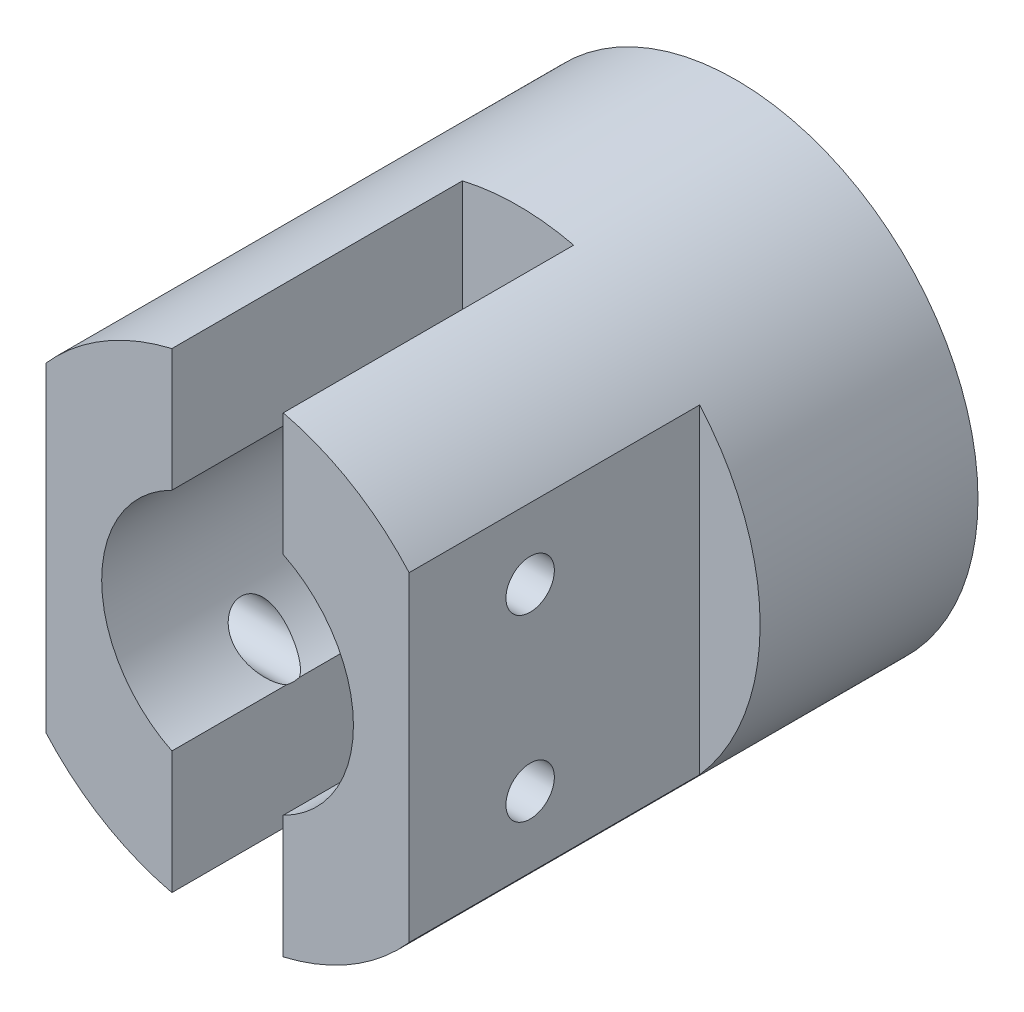
from build123d import *

# Parameters (mm, degrees)
SKETCH2_R           = 5
BOSS_EXTRUDE1_DEPTH = 10.5
SKETCH3_R           = 2.5
CUT_EXTRUDE1_DEPTH  = 3.5
SKETCH4_R           = 1
CUT_EXTRUDE2_DEPTH  = 10.949874371
SKETCH5_W           = 1.25
SKETCH5_H           = 6
CUT_EXTRUDE3_DEPTH  = 16.33786165
SKETCH6_W           = 2.3
SKETCH6_H           = 6
CUT_EXTRUDE4_DEPTH  = 16.33786165
SKETCH7_R           = 2.6
CUT_EXTRUDE5_DEPTH  = 6
SKETCH8_R           = 0.5
CUT_EXTRUDE6_DEPTH  = 15.553779578


with BuildPart() as part:
    # Sketch2 → Boss-Extrude1 (new body)
    with BuildSketch(Plane.XY):
        with Locations(Location((0, 0, 0), (0, 0, 180))):
            Circle(SKETCH2_R)
    extrude(amount=BOSS_EXTRUDE1_DEPTH)

    # Sketch3 → Cut-Extrude1 (cut)
    with BuildSketch(Plane(origin=(0, 0, 0), x_dir=(-1, 0, 0), z_dir=(0, 0, -1))):
        Circle(SKETCH3_R)
    extrude(amount=-CUT_EXTRUDE1_DEPTH, mode=Mode.SUBTRACT)

    # Sketch4 → Cut-Extrude2 (cut, through all)
    with BuildSketch(Plane(origin=(0, 0, 3.5), x_dir=(-1, 0, 0), z_dir=(0, 0, -1))):
        Circle(SKETCH4_R)
    extrude(amount=-CUT_EXTRUDE2_DEPTH, mode=Mode.SUBTRACT)

    # Sketch5 → Cut-Extrude3 (cut, through all)
    with BuildSketch(Plane(origin=(0, 5, 0), x_dir=(1, 0, 0), z_dir=(0, 1, 0))):
        with Locations((-4.375, -7.5)):
            Rectangle(SKETCH5_W, SKETCH5_H)
        with Locations((4.375, -7.5)):
            Rectangle(SKETCH5_W, SKETCH5_H)
    extrude(amount=-CUT_EXTRUDE3_DEPTH, mode=Mode.SUBTRACT)

    # Sketch6 → Cut-Extrude4 (cut, through all)
    with BuildSketch(Plane(origin=(0, 5, 0), x_dir=(1, 0, 0), z_dir=(0, 1, 0))):
        with Locations((0, -7.5)):
            Rectangle(SKETCH6_W, SKETCH6_H)
    extrude(amount=-CUT_EXTRUDE4_DEPTH, mode=Mode.SUBTRACT)

    # Sketch7 → Cut-Extrude5 (cut)
    with BuildSketch(Plane.XY.offset(10.5)):
        Circle(SKETCH7_R)
    extrude(amount=-CUT_EXTRUDE5_DEPTH, mode=Mode.SUBTRACT)

    # Sketch8 → Cut-Extrude6 (cut, through all)
    with BuildSketch(Plane.ZY.offset(3.75)):
        with Locations((8, 1.85)):
            Circle(SKETCH8_R)
        with Locations((8, -1.85)):
            Circle(SKETCH8_R)
    extrude(amount=-CUT_EXTRUDE6_DEPTH, mode=Mode.SUBTRACT)


solid = part.part
